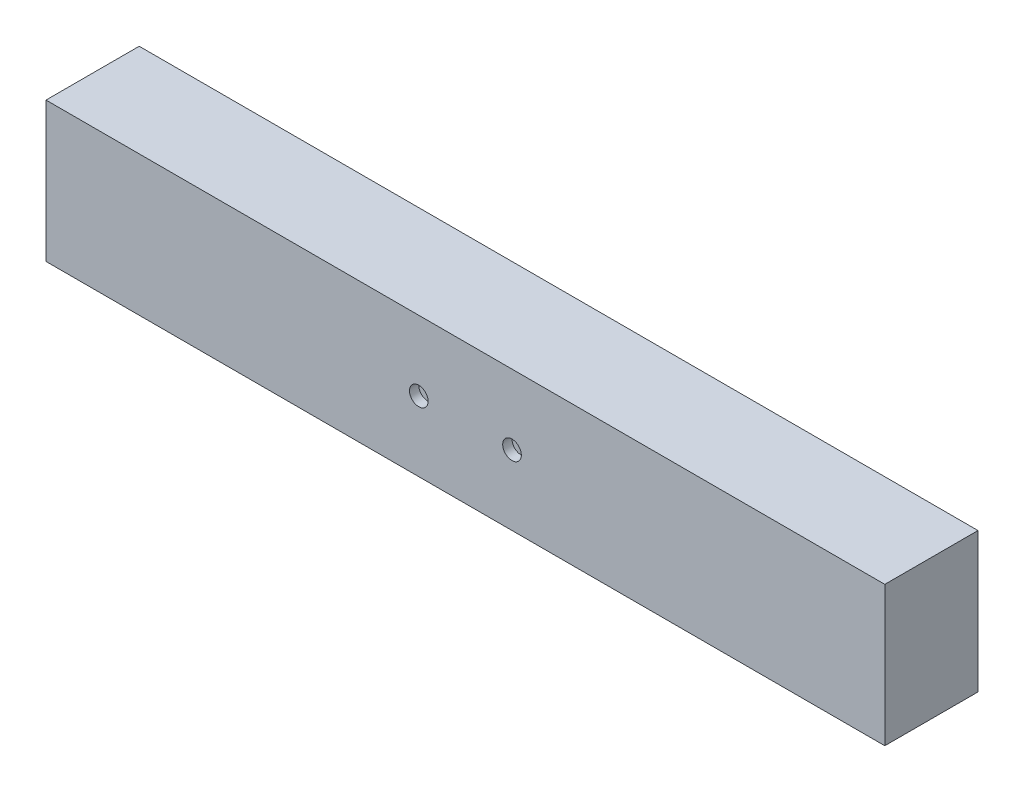
from build123d import *

# Parameters (mm, degrees)
SKETCH_1_W          = 180
SKETCH_1_H          = 30
EXTRUDE_1_DEPTH     = 20
SKETCH_2_R          = 2
CUT_EXTRUDE_1_DEPTH = 2


with BuildPart() as part:
    # 草图1 → 凸台-拉伸1 (new body)
    with BuildSketch(Plane.XY):
        Rectangle(SKETCH_1_W, SKETCH_1_H)
    extrude(amount=EXTRUDE_1_DEPTH)

    # 草图2 → 切除-拉伸1 (cut)
    with BuildSketch(Plane.XY.offset(20)):
        with Locations((-10, 0)):
            Circle(SKETCH_2_R)
        with Locations((10, 0)):
            Circle(SKETCH_2_R)
    extrude(amount=-CUT_EXTRUDE_1_DEPTH, mode=Mode.SUBTRACT)


solid = part.part
